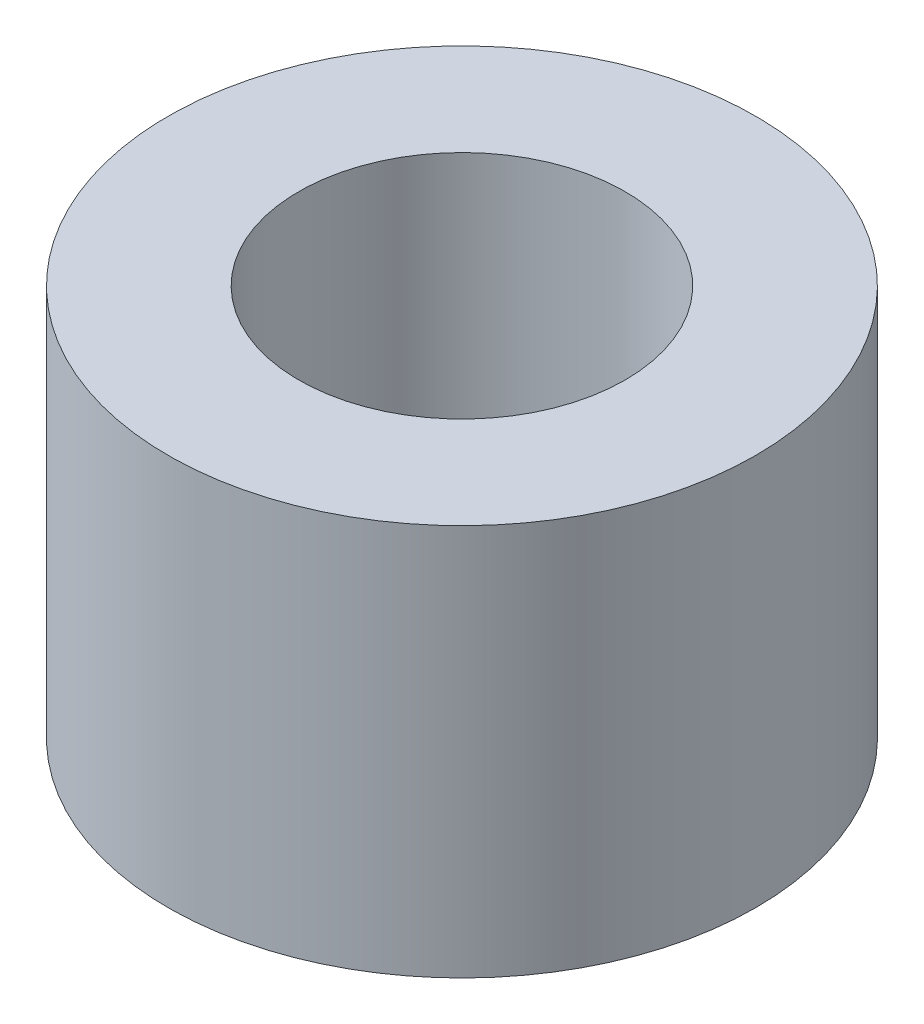
from build123d import *

# Parameters (mm, degrees)
SKETCH1_W = 4
SKETCH1_H = 12


with BuildPart() as part:
    # Sketch1 → Revolve1 (revolve)
    with BuildSketch(Plane.XY):
        with Locations((7, 6)):
            Rectangle(SKETCH1_W, SKETCH1_H)
    revolve(axis=Axis((0, -483.483771846, 0), (0, 1, 0)))


solid = part.part
